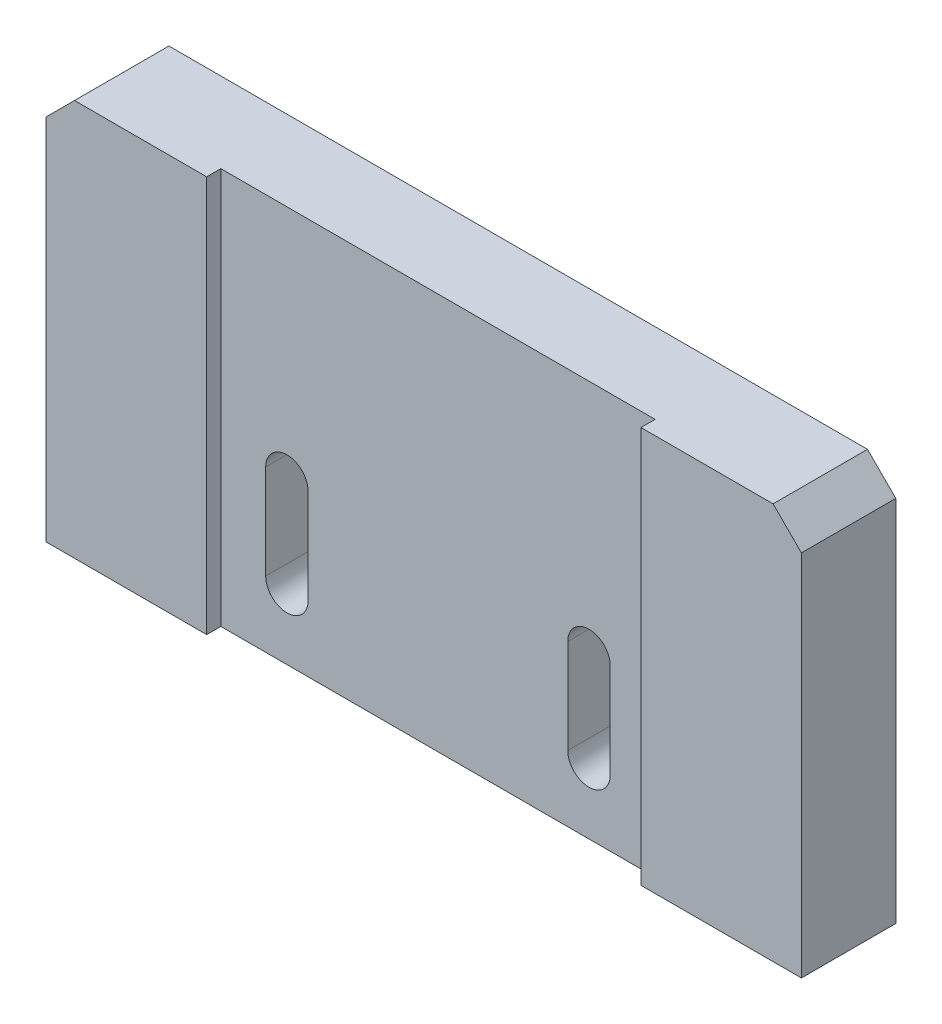
from build123d import *

# Parameters (mm, degrees)
SKETCH_1_W          = 80
SKETCH_1_H          = 42
EXTRUDE_1_DEPTH     = 10
SKETCH_2_W          = 46
SKETCH_2_H          = 42
CUT_EXTRUDE_1_DEPTH = 1.5
CHAMFER_1_SIZE      = 3
CUT_EXTRUDE_2_REACH = 47.97


with BuildPart() as part:
    # 草图1 → 凸台-拉伸1 (new body)
    with BuildSketch(Plane.XY):
        Rectangle(SKETCH_1_W, SKETCH_1_H)
    extrude(amount=EXTRUDE_1_DEPTH)

    # 草图2 → 切除-拉伸1 (cut)
    with BuildSketch(Plane.XY.offset(10)):
        Rectangle(SKETCH_2_W, SKETCH_2_H)
    extrude(amount=-CUT_EXTRUDE_1_DEPTH, mode=Mode.SUBTRACT)

    # 倒角1
    chamfer_1_edges = [part.edges().sort_by_distance(p)[0] for p in [
        (-40, 21, 5),
        (40, 21, 5),
    ]]
    chamfer(chamfer_1_edges, length=CHAMFER_1_SIZE)

    # 草图3 → 切除-拉伸2 (cut, up to next)
    with BuildSketch(Plane.XY.offset(8.5), mode=Mode.PRIVATE) as cut_extrude_2_sk1:
        with BuildLine():
            Line((-18.25, -14), (-18.25, -4))
            ThreePointArc((-18.25, -4), (-16, -1.75), (-13.75, -4))
            Line((-13.75, -4), (-13.75, -14))
            ThreePointArc((-13.75, -14), (-16, -16.25), (-18.25, -14))
        make_face()
    cut_extrude_2_tool1 = extrude(cut_extrude_2_sk1.sketch, amount=-CUT_EXTRUDE_2_REACH, mode=Mode.PRIVATE) & part.part
    cut_extrude_2 = cut_extrude_2_tool1.solids().sort_by_distance((-16, -9, 8.5))[0]
    add(cut_extrude_2, mode=Mode.SUBTRACT)

    # 镜向1: 切除-拉伸2 across plane
    add(cut_extrude_2.mirror(Plane(origin=(0, 0, 0), x_dir=(0, 0, 1), z_dir=(1, 0, 0))), mode=Mode.SUBTRACT)


solid = part.part
